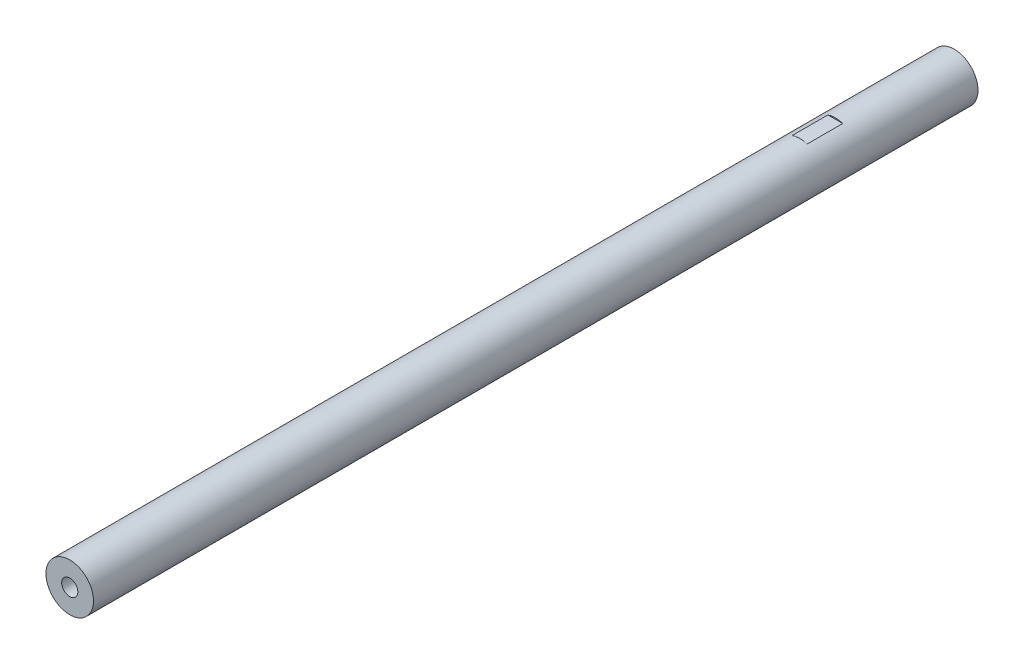
from build123d import *

# Parameters (mm, degrees)
SKETCH1_R             = 10
BOSS_EXTRUDE1_DEPTH   = 186
CUT_EXTRUDE1_START    = -65
CUT_EXTRUDE1_DEPTH    = 15
M8_TAPPED_HOLE1_D     = 6.8
M8_TAPPED_HOLE1_DEPTH = 19.75
M8_TAPPED_HOLE1_TIP   = 2.042926105
M8_TAPPED_HOLE2_D     = 6.8
M8_TAPPED_HOLE2_DEPTH = 19.75
M8_TAPPED_HOLE2_TIP   = 2.042926105


with BuildPart() as part:
    # Sketch1 → Boss-Extrude1 (new, symmetric)
    with BuildSketch(Plane.XY):
        with Locations(Location((0, 0, 0), (0, 0, 180))):
            Circle(SKETCH1_R)
    extrude(amount=BOSS_EXTRUDE1_DEPTH, both=True)

    # Sketch2 → Cut-Extrude1 (cut)
    with BuildSketch(Plane(origin=(0, 0, -186), x_dir=(-1, 0, 0), z_dir=(0, 0, -1)).offset(CUT_EXTRUDE1_START)):
        with BuildLine():
            Line((-3.122498999, -9.5), (3.122498999, -9.5))
            ThreePointArc((3.122498999, -9.5), (0, -10), (-3.122498999, -9.5))
        make_face()
        with BuildLine():
            Line((-3.122498999, 9.5), (3.122498999, 9.5))
            ThreePointArc((3.122498999, 9.5), (0, 10), (-3.122498999, 9.5))
        make_face()
    extrude(amount=CUT_EXTRUDE1_DEPTH, mode=Mode.SUBTRACT)

    # M8 Tapped Hole1
    with Locations(Plane(origin=(0, 0, -186), x_dir=(-1, 0, 0), z_dir=(0, 0, -1))):
        with Locations((0, 0)):
            Hole(M8_TAPPED_HOLE1_D / 2, depth=M8_TAPPED_HOLE1_DEPTH)
            with Locations((0, 0, -(M8_TAPPED_HOLE1_DEPTH + M8_TAPPED_HOLE1_TIP / 2))):  # 118° drill point
                Cone(0, M8_TAPPED_HOLE1_D / 2, M8_TAPPED_HOLE1_TIP, mode=Mode.SUBTRACT)

    # M8 Tapped Hole2
    with Locations(Plane.XY.offset(186)):
        with Locations((0, 0)):
            Hole(M8_TAPPED_HOLE2_D / 2, depth=M8_TAPPED_HOLE2_DEPTH)
            with Locations((0, 0, -(M8_TAPPED_HOLE2_DEPTH + M8_TAPPED_HOLE2_TIP / 2))):  # 118° drill point
                Cone(0, M8_TAPPED_HOLE2_D / 2, M8_TAPPED_HOLE2_TIP, mode=Mode.SUBTRACT)


solid = part.part
